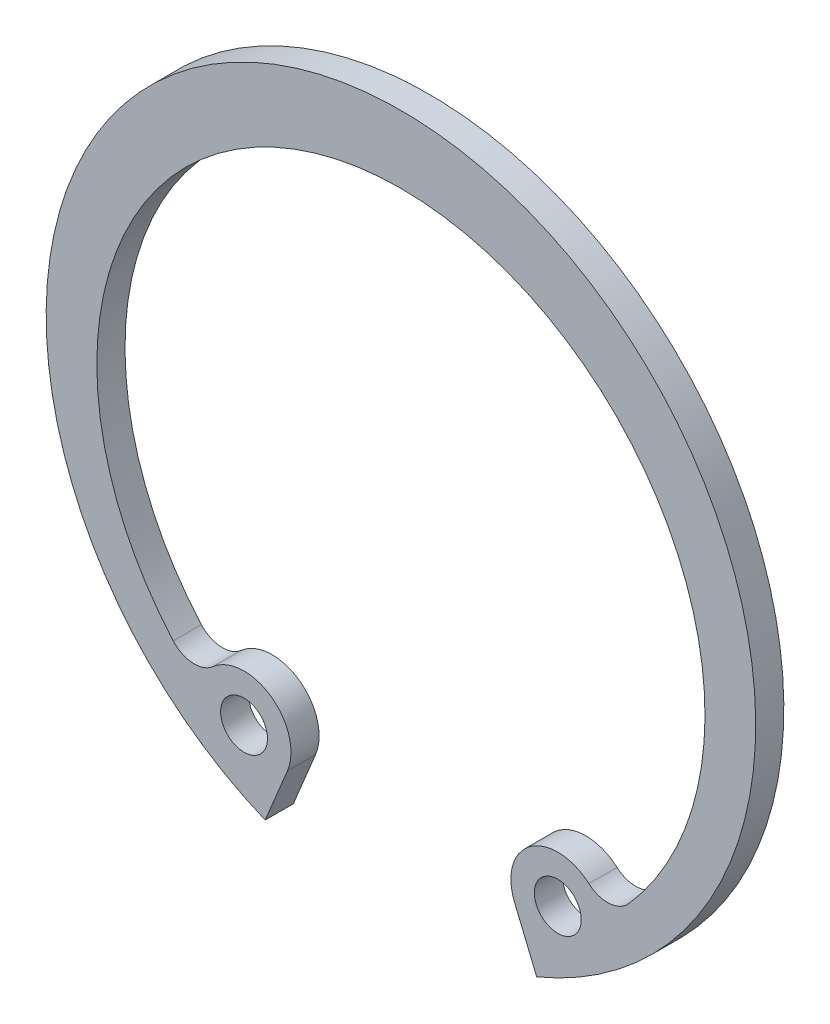
from build123d import *

# Parameters (mm, degrees)
SKETCH1_R  = 1.25
BODY_DEPTH = 1.5


with BuildPart() as part:
    # Sketch1 → Body (new body)
    with BuildSketch(Plane.XY):
        with BuildLine():
            Line((6.047730211, -14.600512296), (7.232716872, -17.461323164))
            ThreePointArc((7.232716872, -17.461323164), (0, 18.9), (-7.232716872, -17.461323164))
            Line((-7.232716872, -17.461323164), (-6.047730211, -14.600512296))
            ThreePointArc((-6.047730211, -14.600512296), (-6.904744304, -11.609176709), (-10.012271945, -11.769905381))
            ThreePointArc((-10.012271945, -11.769905381), (-11.097089224, -12.142747822), (-12.128155002, -11.64001193))
            ThreePointArc((-12.128155002, -11.64001193), (0, 15.3), (12.128155002, -11.64001193))
            ThreePointArc((12.128155002, -11.64001193), (11.097089224, -12.142747822), (10.012271945, -11.769905381))
            ThreePointArc((10.012271945, -11.769905381), (6.904744304, -11.609176709), (6.047730211, -14.600512296))
        make_face()
        with Locations(Location((8.357429042, -13.643803715, 0), (0, 0, 180))):
            Circle(SKETCH1_R, mode=Mode.SUBTRACT)
        with Locations((-8.357429042, -13.643803715)):
            Circle(SKETCH1_R, mode=Mode.SUBTRACT)
    extrude(amount=-BODY_DEPTH)


solid = part.part
